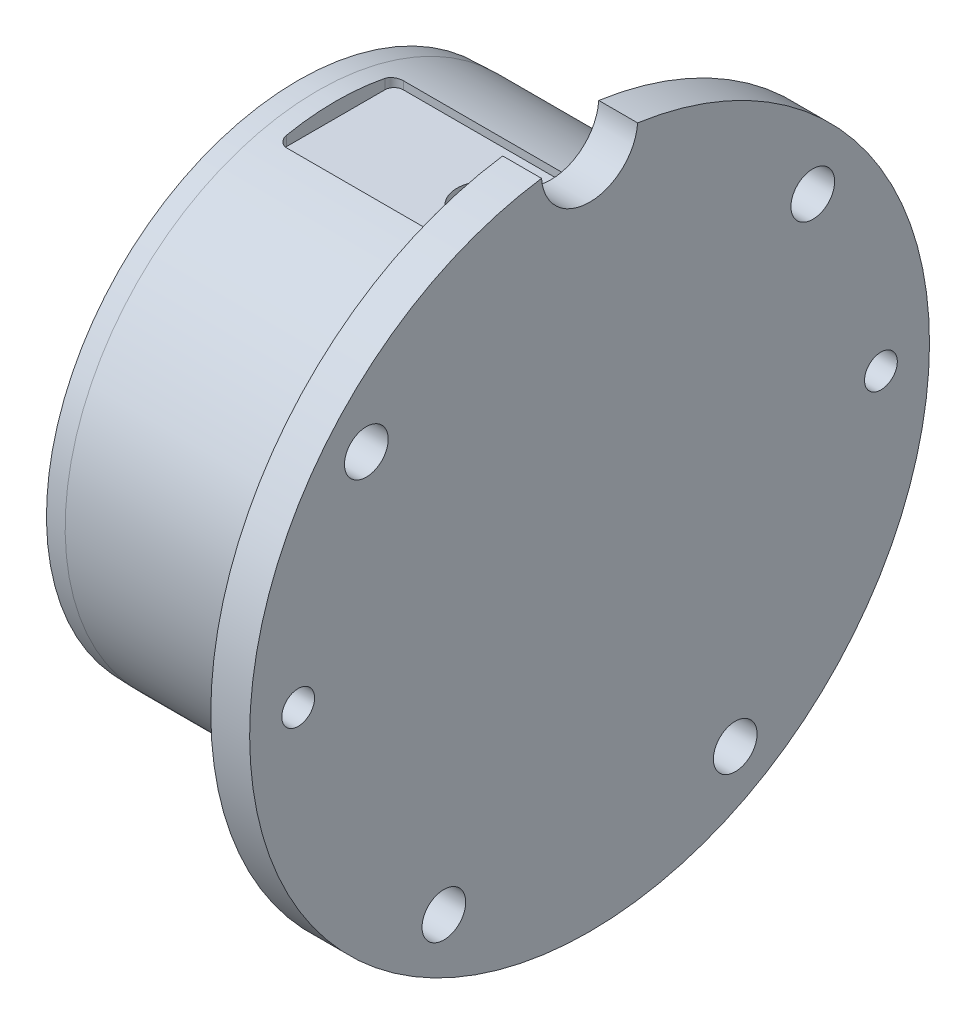
from build123d import *

# Parameters (mm, degrees)
F_9_16_0_5625_DIAMETER_HOLE1_D = 14.2875
F_1_2_13_TAPPED_HOLE1_D        = 10.71626
EXTRUDE1_START                 = 77.724
SKETCH8_W                      = 58.674
SKETCH8_H                      = 38.1
EXTRUDE1_DEPTH                 = 4.8133
EXTRUDE2_REACH                 = 240.925
EXTRUDE2_END_RADIUS            = 65.913
SKETCH9_R                      = 9.525
FILLET1_R                      = 3
EXTRUDE3_REACH                 = 185.766


with BuildPart() as part:
    # Sketch1 → Revolve1 (revolve)
    with BuildSketch(Plane.XY):
        Polygon((-95.25, 70.620031854), (-95.25, 82.2956), (-88.9, 82.5373), (-12.7, 82.5373), (-12.7, 111.125), (0, 111.125), (0, 0), (-24.2804, 0), (-24.2804, 65.913), (-40.0304, 65.913), (-40.0304, 70.0075), (-88.4682, 70.0075), (-88.4682, 73.279), (-91.5162, 73.279), (-91.5162, 70.0075), (-92.964, 70.0075), align=None)
    revolve(axis=Axis((0, 0, 0), (-1, 0, 0)))

    # 9/16 (0.5625) Diameter Hole1 (through all)
    with Locations(Plane(origin=(0, 0, 0), x_dir=(0, 0, -1), z_dir=(1, 0, 0))):
        with Locations((-72.9742, 61.2154), (72.9742, 61.2154), (-47.625, -82.4992), (47.625, -82.4992)):
            Hole(F_9_16_0_5625_DIAMETER_HOLE1_D / 2)

    # 1/2-13 Tapped Hole1 (through all)
    with Locations(Plane(origin=(0, 0, 0), x_dir=(0, 0, -1), z_dir=(1, 0, 0))):
        with Locations((-95.25, 0), (95.25, 0)):
            Hole(F_1_2_13_TAPPED_HOLE1_D / 2)

    # Sketch8 → Extrude1 (cut)
    with BuildSketch(Plane(origin=(0, 0, 0), x_dir=(1, 0, 0), z_dir=(0, 1, 0)).offset(EXTRUDE1_START)):
        with Locations((-53.6174, 0)):
            Rectangle(SKETCH8_W, SKETCH8_H)
    extrude(amount=EXTRUDE1_DEPTH, mode=Mode.SUBTRACT)

    # Extrude2: up to this cylinder (the profile starts outside it)
    extrude2_end = Plane(origin=(-33.8054, 0, 0), z_dir=(1, 0, 0)) * Cylinder(EXTRUDE2_END_RADIUS, 614.676, mode=Mode.PRIVATE)
    # Sketch9 → Extrude2 (cut, up to the surface)
    with BuildSketch(Plane(origin=(0, 77.724, 0), x_dir=(1, 0, 0), z_dir=(0, 1, 0)), mode=Mode.PRIVATE) as extrude2_sk1:
        with Locations((-33.8054, 0)):
            Circle(SKETCH9_R)
    extrude2_tool1 = extrude(extrude2_sk1.sketch, amount=-EXTRUDE2_REACH, mode=Mode.PRIVATE) - extrude2_end
    add(extrude2_tool1.solids().sort_by_distance((-33.8054, 77.724, 0))[0], mode=Mode.SUBTRACT)

    # Fillet1
    fillet1_edges = [part.edges().sort_by_distance(p)[0] for p in [
        (-82.9544, 79.016400105, 19.05),
        (-82.9544, 79.016400105, -19.05),
    ]]
    fillet(fillet1_edges, radius=FILLET1_R)

    # Sketch10 → Extrude3 (cut, up to next)
    with BuildSketch(Plane(origin=(0, 0, 0), x_dir=(0, 0, -1), z_dir=(1, 0, 0)), mode=Mode.PRIVATE) as extrude3_sk1:
        with BuildLine():
            ThreePointArc((-15.708416989, 110.009141714), (0, 95.377), (15.708416989, 110.009141714))
            ThreePointArc((15.708416989, 110.009141714), (0, 111.125), (-15.708416989, 110.009141714))
        make_face()
    extrude3_tool1 = extrude(extrude3_sk1.sketch, amount=-EXTRUDE3_REACH, mode=Mode.PRIVATE) & part.part
    add(extrude3_tool1.solids().sort_by_distance((0, 104.244395, 0))[0], mode=Mode.SUBTRACT)


solid = part.part
